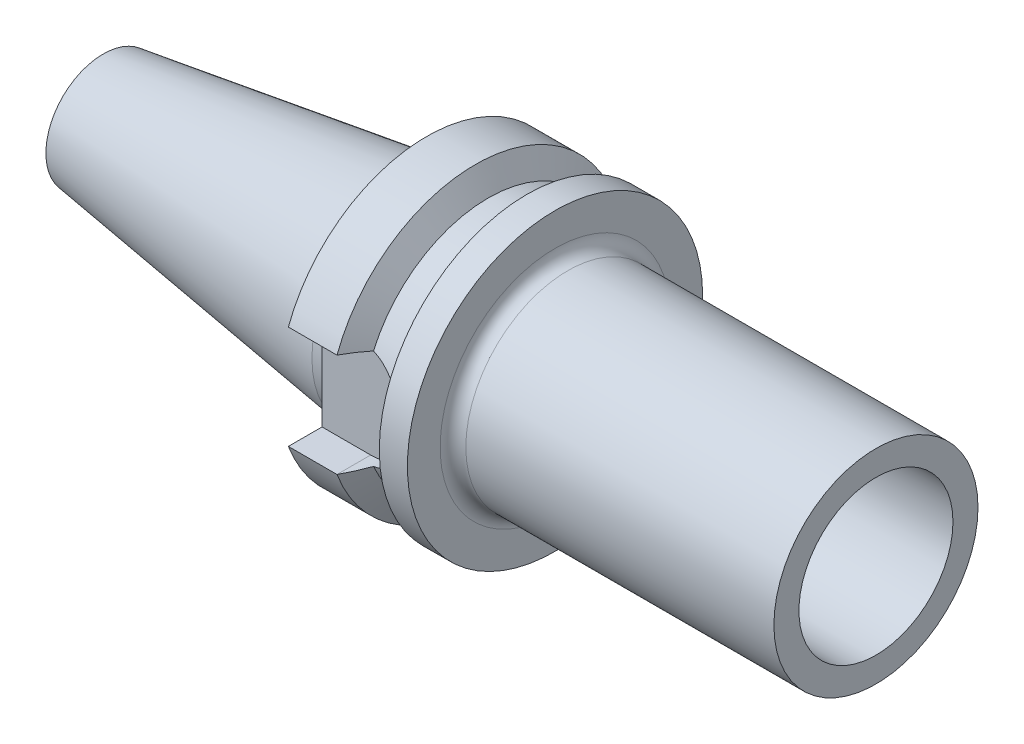
from build123d import *

# Parameters (mm, degrees)
CUT_EXTRUDE_1_DEPTH = 10
SKETCH_4_R          = 15.9
EXTRUDE_1_DEPTH     = 50
FILLET_1_R          = 2
SKETCH_5_R          = 6
CUT_EXTRUDE_2_DEPTH = 125.716318135
SKETCH_6_R          = 12
CUT_EXTRUDE_3_DEPTH = 30
SKETCH_7_R          = 3
EXTRUDE_2_DEPTH     = 6


with BuildPart() as part:
    # 草图1 → 旋转1 (revolve)
    with BuildSketch(Plane.XY, mode=Mode.PRIVATE) as revolve_1_sk:
        Polygon((0, 0), (0, 8.92200912), (48.4, 15.875), (50.4, 15.875), (50.4, 23), (57.979274058, 23), (60, 19.5), (64, 19.5), (66.020725942, 23), (70.4, 23), (70.4, 0), align=None)
    revolve(revolve_1_sk.sketch.rotate(Axis((70.4, 0, 0), (-1, 0, 0)), 90), axis=Axis((70.4, 0, 0), (-1, 0, 0)))

    # 草图2 → 切除-拉伸1 (cut)
    with BuildSketch(Plane.XY.offset(16.3)):
        with BuildLine():
            Line((57.979274058, 8.05), (50.4, 8.05))
            Line((50.4, 8.05), (50.4, -8.05))
            Line((50.4, -8.05), (57.979274058, -8.05))
            ThreePointArc((57.979274058, -8.05), (66.029274058, 0), (57.979274058, 8.05))
        make_face()
    cut_extrude_1 = extrude(amount=CUT_EXTRUDE_1_DEPTH, mode=Mode.SUBTRACT)

    # 镜向1: 切除-拉伸1 across plane
    add(cut_extrude_1.mirror(Plane.XY), mode=Mode.SUBTRACT)

    # 草图4 → 凸台-拉伸1 (add)
    with BuildSketch(Plane(origin=(70.4, 0, 0), x_dir=(0, 0, -1), z_dir=(1, 0, 0))):
        Circle(SKETCH_4_R)
    extrude(amount=EXTRUDE_1_DEPTH)

    # 圆角1
    fillet_1_edges = [part.edges().sort_by_distance(p)[0] for p in [
        (70.4, 0, 15.9),
    ]]
    fillet(fillet_1_edges, radius=FILLET_1_R)

    # 草图5 → 切除-拉伸2 (cut, through all)
    with BuildSketch(Plane.ZY):
        Circle(SKETCH_5_R)
    extrude(amount=-CUT_EXTRUDE_2_DEPTH, mode=Mode.SUBTRACT)

    # 草图6 → 切除-拉伸3 (cut)
    with BuildSketch(Plane(origin=(120.4, 0, 0), x_dir=(0, 0, -1), z_dir=(1, 0, 0))):
        Circle(SKETCH_6_R)
    extrude(amount=-CUT_EXTRUDE_3_DEPTH, mode=Mode.SUBTRACT)


with BuildPart() as body_2:
    # 草图7 → 凸台-拉伸2 (new body)
    with BuildSketch(Plane.ZY.offset(-50.4)):
        Circle(SKETCH_7_R)
    extrude(amount=-EXTRUDE_2_DEPTH)


solid = Compound([part.part, body_2.part])
